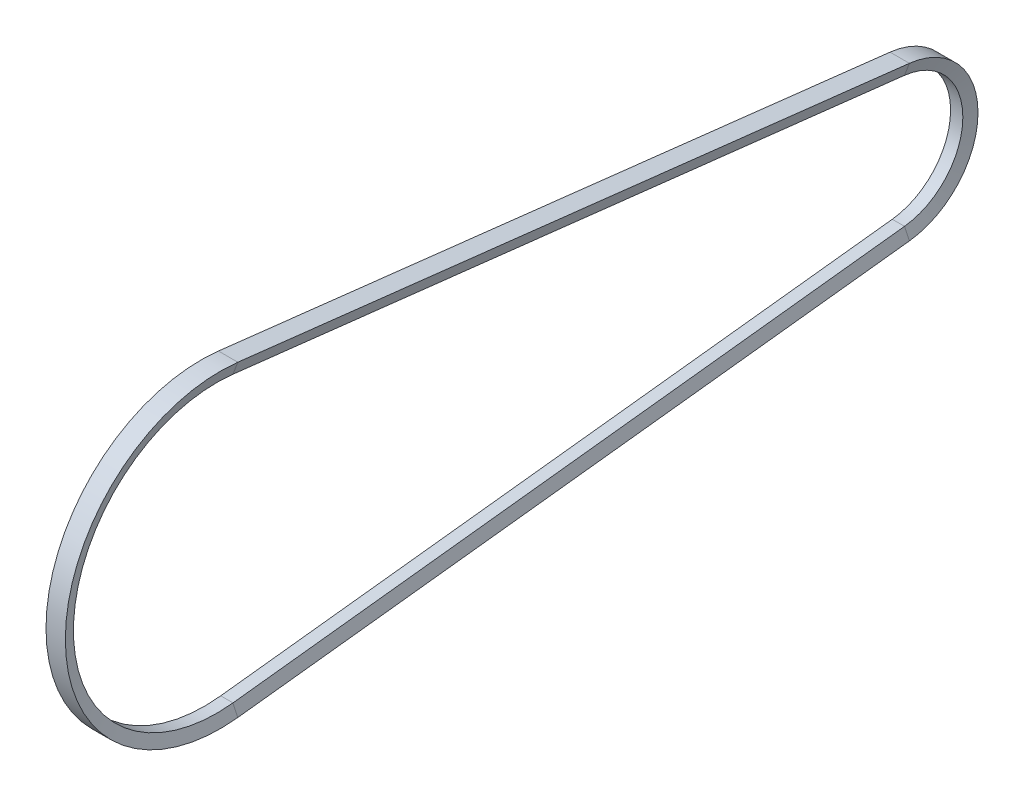
from build123d import *


with BuildPart() as part:
    # 扫描1: sweep along a path in 草图1
    with BuildLine(Plane(origin=(0, 0, 0), x_dir=(0, 0, -1), z_dir=(1, 0, 0))) as sweep_1_path:
        Line((9.103840683, 79.480312561), (356.051920341, 39.740156281))
        ThreePointArc((356.051920341, 39.740156281), (391.5, 0), (356.051920341, -39.740156281))
        Line((356.051920341, -39.740156281), (9.103840683, -79.480312561))
        ThreePointArc((9.103840683, -79.480312561), (-80, 0), (9.103840683, 79.480312561))
    # 草图2 → 扫描1 (sweep)
    with BuildSketch(Plane.XY):
        Polygon((-5, 80), (5, 80), (3.165615911, 74), (-3.165615911, 74), align=None)
    sweep(path=sweep_1_path.line)


solid = part.part
